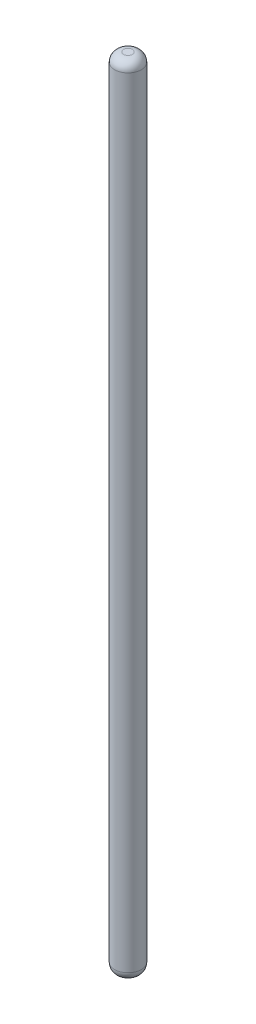
SolidWorks part; units mm, degrees
ref_plane "Front Plane" through (0, 0, 0) normal (0, 0, 1) x (1, 0, 0)
ref_plane "Top Plane" through (0, 0, 0) normal (0, 1, 0) x (1, 0, 0)
ref_plane "Right Plane" through (0, 0, 0) normal (1, 0, 0) x (0, 0, -1)
sketch "Sketch1" plane through (0, 0, 0) normal (0, 1, 0) x (1, 0, 0)
  circle A0 centre (0, 0) radius 3
  dimension "D1" = 6
extrude "Boss-Extrude1" add sketch "Sketch1" along normal blind 180
fillet "Fillet1" radius 2 2 edges at (0, 0, 3) (0, 180, 3)
